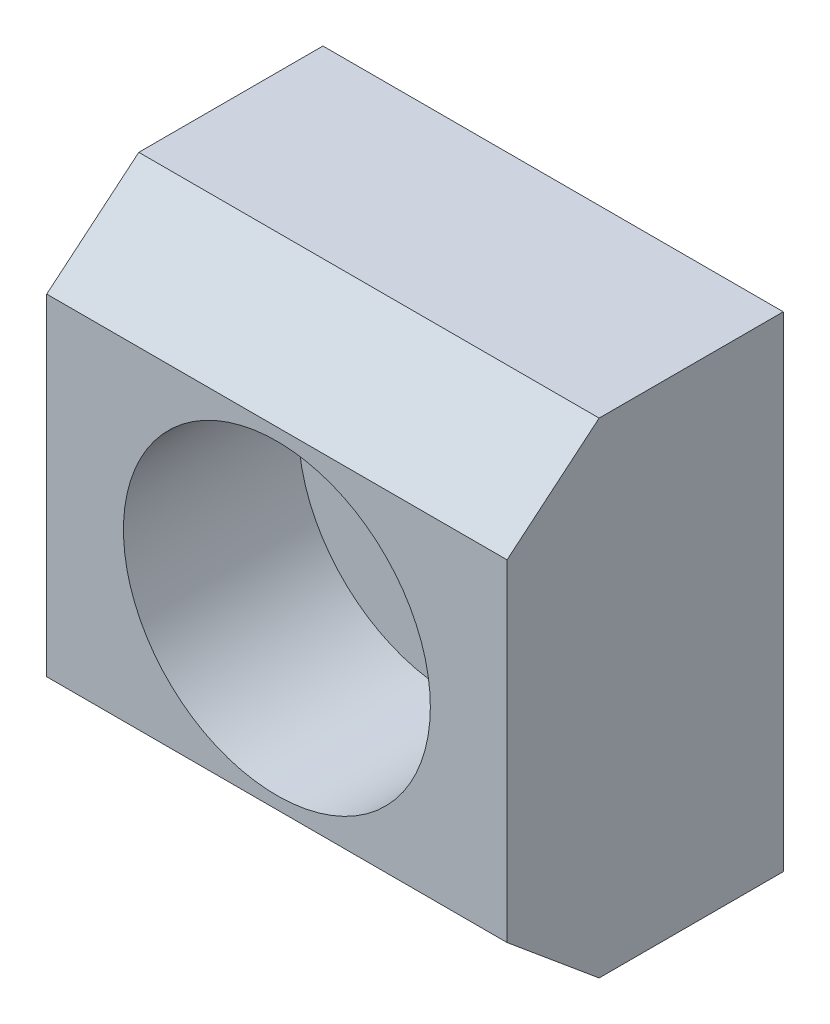
from build123d import *

# Parameters (mm, degrees)
SKETCH_1_W                   = 15
SKETCH_1_H                   = 15.8
EXTRUDE_1_DEPTH              = 4.5
HOLE_WIZARD_M4_1_D           = 5.5
HOLE_WIZARD_M4_1_CBORE_D     = 10
HOLE_WIZARD_M4_1_CBORE_DEPTH = 5.7
CUT_EXTRUDE_1_DEPTH          = 18.540239451


with BuildPart() as part:
    # 草图1 → 凸台-拉伸1 (new, symmetric)
    with BuildSketch(Plane.XY):
        Rectangle(SKETCH_1_W, SKETCH_1_H)
    extrude(amount=EXTRUDE_1_DEPTH, both=True)

    # M4 沉头孔1 (through all)
    with Locations(Plane.XY.offset(4.5)):
        with Locations((0, 0)):
            CounterBoreHole(HOLE_WIZARD_M4_1_D / 2, HOLE_WIZARD_M4_1_CBORE_D / 2, HOLE_WIZARD_M4_1_CBORE_DEPTH)

    # 草图4 → 切除-拉伸1 (cut, through all)
    with BuildSketch(Plane(origin=(7.5, 0, 0), x_dir=(0, 0, -1), z_dir=(1, 0, 0))):
        Polygon((-4.5, -7.9), (-4.5, -5.4), (-1.5, -7.9), align=None)
        Polygon((-4.5, 5.4), (-4.5, 7.9), (-1.5, 7.9), align=None)
    extrude(amount=-CUT_EXTRUDE_1_DEPTH, mode=Mode.SUBTRACT)


solid = part.part
